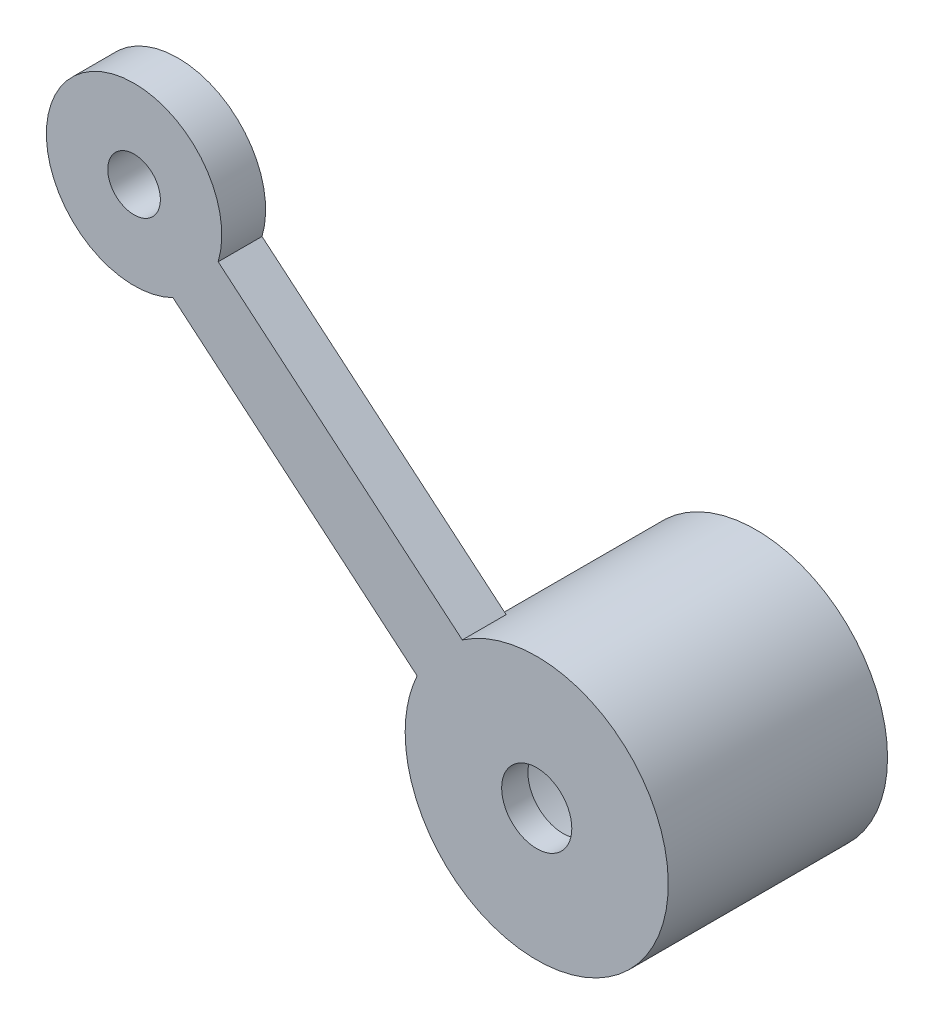
SolidWorks part; units mm, degrees
ref_plane "Front Plane" through (0, 0, 0) normal (0, 0, 1) x (1, 0, 0)
ref_plane "Top Plane" through (0, 0, 0) normal (0, 1, 0) x (1, 0, 0)
ref_plane "Right Plane" through (0, 0, 0) normal (1, 0, 0) x (0, 0, -1)
sketch "Sketch1" plane through (0, 0, 0) normal (0, 0, 1) x (1, 0, 0)
  line L0 (0, 0) -> (45.9099, -38.63) construction
  line L1 (4.4375, -8.9615) -> (32.2727, -32.3829)
  line L2 (9.5882, -2.8402) -> (37.4234, -26.2616)
  circle A0 centre (0, 0) radius 3
  arc A1 (9.5882, -2.8402) -> (4.4375, -8.9615) centre (0, 0) ccw
  arc A3 (32.2727, -32.3829) -> (37.4234, -26.2616) centre (45.9099, -38.63) ccw
  circle A5 centre (45.9099, -38.63) radius 4
  dimension "D1" = 6
  dimension "D2" = 8
  dimension "D5" = 15
  dimension "D6" = 10
  dimension "D3" = 8
  dimension "D4" = 60
extrude "Boss-Extrude1" add sketch "Sketch1" along normal blind 5
sketch "Sketch2" plane through (0, 0, 0) normal (0, 0, -1) x (-1, 0, 0)
  circle A0 centre (-45.9099, -38.63) radius 13
  dimension "D1" = 26
extrude "Cut-Extrude1" cut sketch "Sketch2" against normal blind 2
sketch "Sketch4" plane through (0, 0, 0) normal (0, 0, -1) x (-1, 0, 0)
  circle A0 centre (-45.9099, -25.63) radius 1.25
  circle A1 centre (-45.9099, -38.63) radius 13 construction
  circle A2 centre (-45.9099, -38.63) radius 13 construction
  circle A3 centre (-57.1683, -45.13) radius 1.25
  circle A4 centre (-34.6516, -45.13) radius 1.25
  point P13 (-45.9099, -38.63)
  dimension "D1" = 2.5
extrude "Boss-Extrude2" add sketch "Sketch4" against normal blind 2
sketch "Sketch5" plane through (0, 0, 0) normal (0, 0, -1) x (-1, 0, 0)
  circle A0 centre (-45.9099, -38.63) radius 15
  circle A1 centre (-45.9099, -38.63) radius 13
extrude "Boss-Extrude3" add sketch "Sketch5" along normal blind 20
